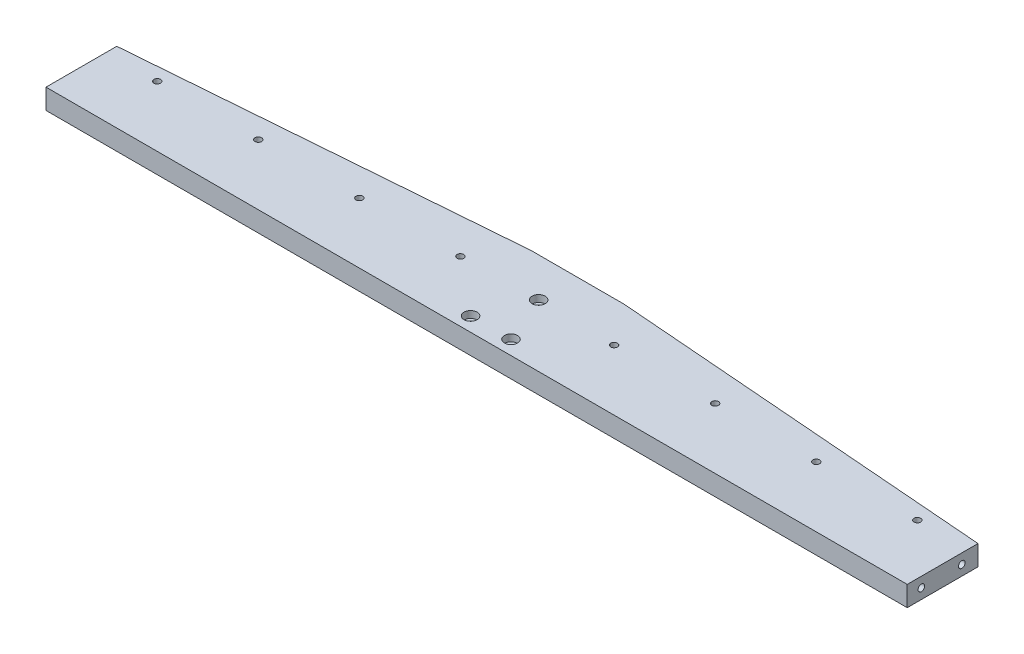
from build123d import *

# Parameters (mm, degrees)
SKETCH_1_W                   = 426
SKETCH_1_H                   = 50
EXTRUDE_1_DEPTH              = 10
HOLE_WIZARD_M4_1_AT_2_COUNT  = 2
HOLE_WIZARD_M4_1_AT_2_PITCH  = 20
HOLE_WIZARD_M3_1_D           = 3.4
HOLE_WIZARD_M3_1_CBORE_D     = 6.5
HOLE_WIZARD_M3_1_CBORE_DEPTH = 3.4
HOLE_WIZARD_M4_2_D           = 3.3
CHAMFER_1_SIZE               = 15
CHAMFER_1_SIZE2              = 190
CHAMFER_2_SIZE               = 190
CHAMFER_2_SIZE2              = 15


with BuildPart() as part:
    # 草图1 → 凸台-拉伸1 (new body)
    with BuildSketch(Plane(origin=(0, 0, 0), x_dir=(1, 0, 0), z_dir=(0, 1, 0))):
        Rectangle(SKETCH_1_W, SKETCH_1_H)
    extrude(amount=EXTRUDE_1_DEPTH)

    # 草图3 → M4 螺纹孔1 (revolve, cut)
    with BuildSketch(Plane(origin=(-213, 5, -2), x_dir=(0, 0, 1), z_dir=(0, 1, 0))):
        Polygon((0, 0), (0, 12.491420021), (1.65, 11.5), (1.65, 0), align=None)
    hole_wizard_m4_1 = revolve(axis=Axis((-219.35, 5, -2), (1, 0, 0)), mode=Mode.SUBTRACT)

    # M4 螺纹孔1 at 2: M4 螺纹孔1 ×2
    with Locations(*[(0, 0, i * HOLE_WIZARD_M4_1_AT_2_PITCH) for i in range(1, HOLE_WIZARD_M4_1_AT_2_COUNT)]):
        add(hole_wizard_m4_1, mode=Mode.SUBTRACT)

    # 镜向1: M4 螺纹孔1 across plane
    add(hole_wizard_m4_1.mirror(Plane(origin=(0, 0, 0), x_dir=(0, 0, 1), z_dir=(1, 0, 0))), mode=Mode.SUBTRACT)

    # 镜向1 copy 1 sketch → 镜向1 copy 1 (revolve, cut)
    with BuildSketch(Plane(origin=(213, 5, 18), x_dir=(0, 0, 1), z_dir=(0, 1, 0))):
        Polygon((0, 0), (0, -12.491420021), (1.65, -11.5), (1.65, 0), align=None)
    revolve(axis=Axis((219.35, 5, 18), (1, 0, 0)), mode=Mode.SUBTRACT)

    # M3 六角凹头螺钉的柱形沉头孔1 (through all)
    with Locations(Plane(origin=(0, 10, 0), x_dir=(1, 0, 0), z_dir=(0, 1, 0))):
        with Locations((10, -18), (-10, -18), (0, 5.7)):
            CounterBoreHole(HOLE_WIZARD_M3_1_D / 2, HOLE_WIZARD_M3_1_CBORE_D / 2, HOLE_WIZARD_M3_1_CBORE_DEPTH)

    # M4 螺纹孔2 (through all)
    with Locations(Plane(origin=(0, 10, 0), x_dir=(1, 0, 0), z_dir=(0, 1, 0))):
        with Locations((-38, 5), (-88, 5), (-138, 5), (-188, 5)):
            hole_wizard_m4_2 = Hole(HOLE_WIZARD_M4_2_D / 2)

    # 镜向2: M4 螺纹孔2 across plane
    add(hole_wizard_m4_2.mirror(Plane(origin=(0, 0, 0), x_dir=(0, 0, 1), z_dir=(1, 0, 0))), mode=Mode.SUBTRACT)

    # 倒角1
    chamfer_1_edges = [part.edges().sort_by_distance(p)[0] for p in [
        (213, 5, -25),
    ]]
    chamfer_1_side = [part.faces().sort_by_distance(p)[0] for p in [
        (213, 5, -0.283390906),
    ]]
    chamfer(chamfer_1_edges, length=CHAMFER_1_SIZE, length2=CHAMFER_1_SIZE2, reference=chamfer_1_side[0])

    # 倒角2
    chamfer_2_edges = [part.edges().sort_by_distance(p)[0] for p in [
        (-213, 5, -25),
    ]]
    chamfer_2_side = [part.faces().sort_by_distance(p)[0] for p in [
        (-95, 5, -25),
    ]]
    chamfer(chamfer_2_edges, length=CHAMFER_2_SIZE, length2=CHAMFER_2_SIZE2, reference=chamfer_2_side[0])


solid = part.part
